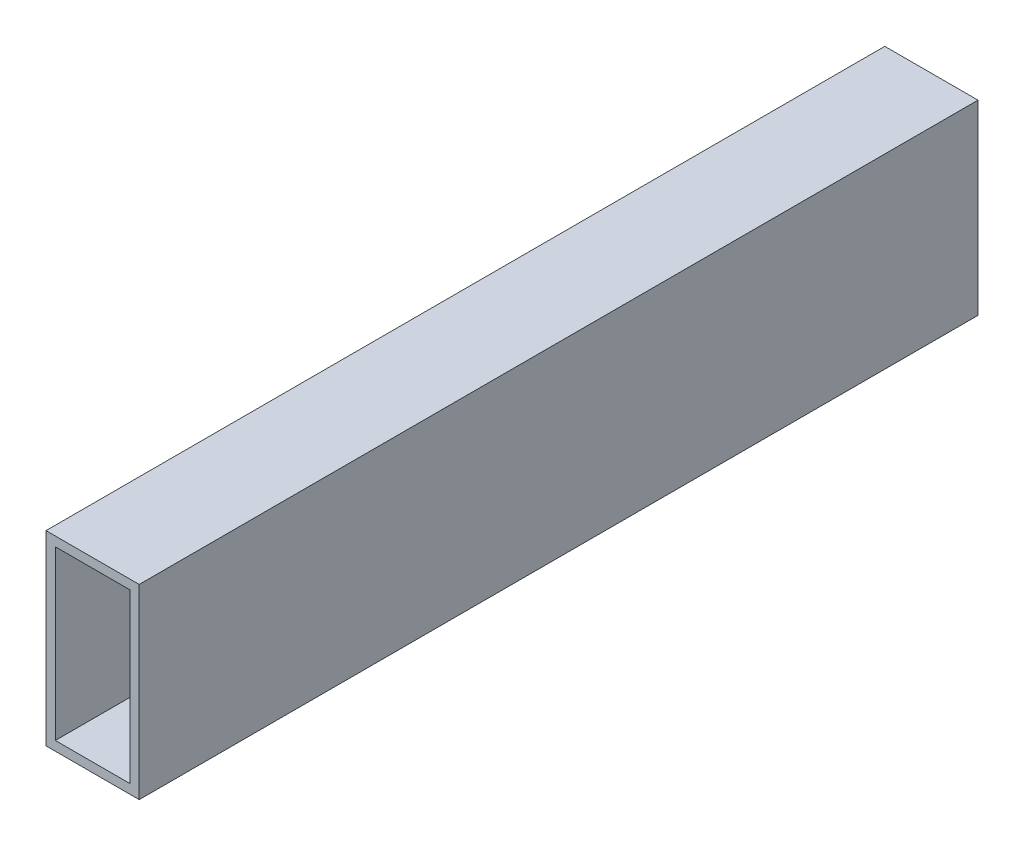
SolidWorks part; units mm, degrees
ref_plane "前视基准面" through (0, 0, 0) normal (0, 0, 1) x (1, 0, 0)
ref_plane "上视基准面" through (0, 0, 0) normal (0, 1, 0) x (1, 0, 0)
ref_plane "右视基准面" through (0, 0, 0) normal (1, 0, 0) x (0, 0, -1)
other "Configuration Table"
sketch "草图1" plane through (0, 0, 0) normal (0, 0, 1) x (1, 0, 0)
  line L0 (-20, -40) -> (20, -40)
  line L1 (20, -40) -> (20, 40)
  line L2 (20, 40) -> (-20, 40)
  line L3 (-20, 40) -> (-20, -40)
  line L4 (-16, -36) -> (16, -36)
  line L5 (16, -36) -> (16, 36)
  line L6 (16, 36) -> (-16, 36)
  line L7 (-16, 36) -> (-16, -36)
  point P0 (0, 0)
  dimension "D1" = 4
  dimension "D2" = 20
  dimension "D3" = 36
  dimension "D4" = 40
  dimension "D5" = 4
  dimension "D6" = 40
  dimension "D7" = 76
  dimension "D8" = 80
extrude "凸台-拉伸1" add sketch "草图1" against normal mid plane 360
